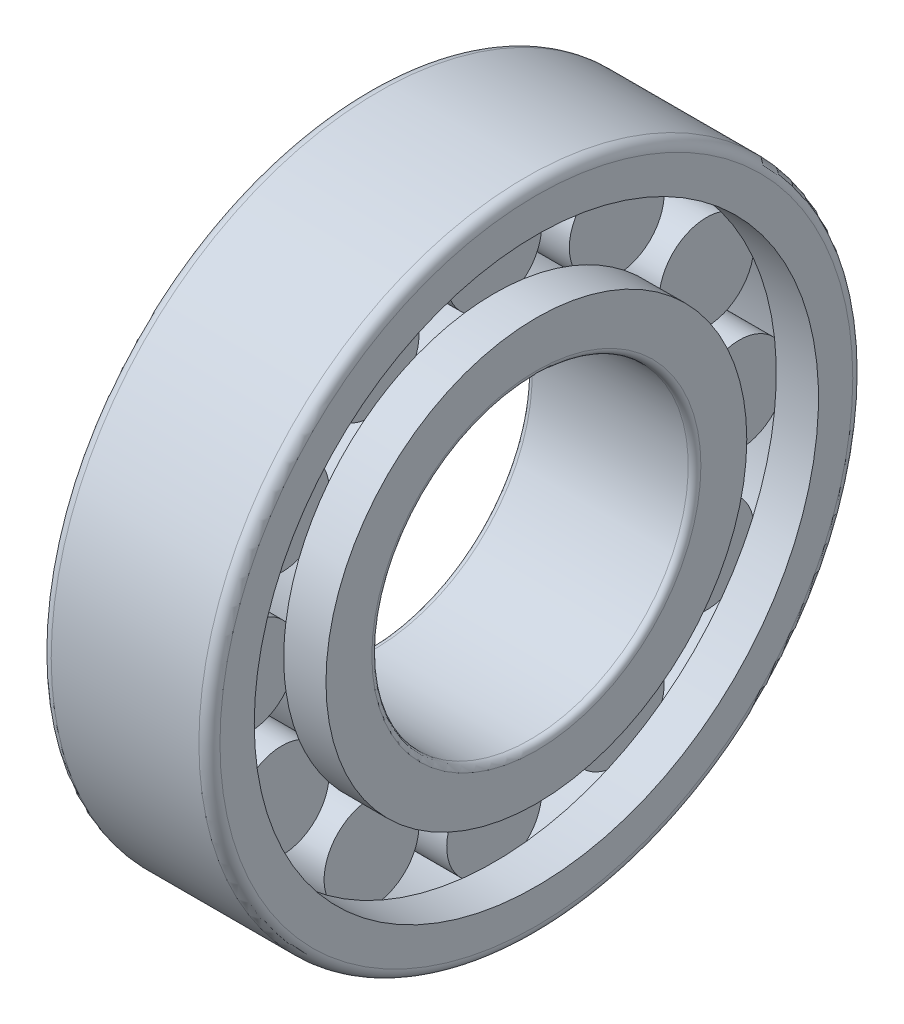
SolidWorks part; units mm, degrees
revolve "基体-旋转" add sketch "草图2" angle 360 about L0
sketch "草图2" plane through (0, 0, 0) normal (0, 0, 1) x (1, 0, 0)
  line L0 (-10.0801, 0) -> (21.9267, 0) construction
  line L1 (4, 18.75) -> (12, 18.75)
  line L2 (0, 19.95) -> (4, 19.95)
  line L3 (0, 19.95) -> (0, 15.6)
  line L4 (0.6, 15) -> (15.4, 15)
  line L5 (16, 19.95) -> (16, 15.6)
  line L6 (4, 18.75) -> (4, 19.95)
  line L7 (12, 18.75) -> (12, 19.95)
  line L8 (12, 19.95) -> (16, 19.95)
  arc A0 (15.4, 15) -> (16, 15.6) centre (15.4, 15.6) ccw
  arc A1 (0, 15.6) -> (0.6, 15) centre (0.6, 15.6) ccw
  point P13 (16, 15)
  point P16 (0, 15)
ref_plane "基准面1" through (0, 0, 0) normal (0, 0, 1) x (1, 0, 0)
ref_plane "基准面2" through (0, 0, 0) normal (0, 1, 0) x (1, 0, 0)
ref_plane "基准面3" through (0, 0, 0) normal (1, 0, 0) x (0, 0, -1)
sketch "尺寸草图" plane through (0, 0, 0) normal (0, 0, 1) x (1, 0, 0)
  line L0 (0, 0) -> (0.6, 0)
  line L1 (0.6, 0) -> (1.6, 0)
  line L2 (1.6, 0) -> (17.6, 0)
  line L3 (17.6, 0) -> (47.6, 0)
  line L4 (47.6, 0) -> (85.1, 0)
  line L5 (85.1, 0) -> (147.1, 0)
  line L7 (147.1, 0) -> (202.6, 0)
sketch "草图3" plane through (0, 0, 0) normal (0, 0, 1) x (1, 0, 0)
  line L0 (12, 19.95) -> (12, -19.95) construction
  line L2 (-1.6039, 23.25) -> (13.5036, 23.25) construction
  line L4 (4, 23.25) -> (12, 23.25)
  line L5 (4, 23.25) -> (4, 18.7499)
  line L6 (4, 18.7499) -> (12, 18.7499)
  line L7 (12, 23.25) -> (12, 18.7499)
  line L8 (4, -19.95) -> (4, 19.95) construction
revolve "凸台-旋转1" add sketch "草图3" angle 360 about L2
sketch "草图4" plane through (0, 0, 0) normal (0, 0, 1) x (1, 0, 0)
  line L0 (0, 0) -> (17.8006, 0) construction
  line L1 (-10.0801, 0) -> (21.9267, 0) construction
  line L2 (12, 26.75) -> (16, 26.75)
  line L3 (1, 31) -> (15, 31)
  line L4 (0, 30) -> (0, 26.75)
  line L5 (0, 26.75) -> (4, 26.75)
  line L6 (16, 30) -> (16, 26.75)
  line L7 (4, 27.75) -> (12, 27.75)
  line L8 (4, 27.75) -> (4, 26.75)
  line L10 (12, 27.75) -> (12, 26.75)
  arc A0 (15, 31) -> (16, 30) centre (15, 30) cw
  arc A1 (1, 31) -> (0, 30) centre (1, 30) ccw
  point P15 (16, 31)
  point P18 (0, 31)
revolve "凸台-旋转2" add sketch "草图4" angle 360 about L0
pattern_circular "阵列(圆周)1" count 12 over 360 about axis through (0, 0, 0) along (1, 0, 0) of "凸台-旋转1"
equation "\"DD@草图2\" = \"内径@尺寸草图\""
equation "\"FW@草图2\" = \"参考FW@尺寸草图\""
equation "\"D1@草图2\" = \"倒角小@尺寸草图\""
equation "\"EW@草图4\" = \"参考EW@尺寸草图\""
equation "\"D@草图4\" = \"外径@尺寸草图\""
equation "\"D2@草图4\" = \"倒角大@尺寸草图\""
equation "\"B@草图4\" = \"宽度@尺寸草图\""
equation "\"D2@草图2\" = \"B@草图4\""
equation "\"滚珠位置@草图2\" = \"D2@草图2\"/4"
equation "\"D3@草图4\" = \"D2@草图4\""
equation "\"D1@草图3\" =  ( \"EW@草图4\" - \"FW@草图2\" )  / 4 + \"FW@草图2\" / 2"
equation "\"D2@草图3\" =  0.25*( \"EW@草图4\" - \"FW@草图2\" ) +0.0001"
equation "\"D4@草图2\" = \"FW@草图2\" + 4 *\"D1@草图2\""
equation "\"D1@阵列(圆周)1\" =0.75* \"D1@草图3\" * 3.14 / \"D2@草图3\""
